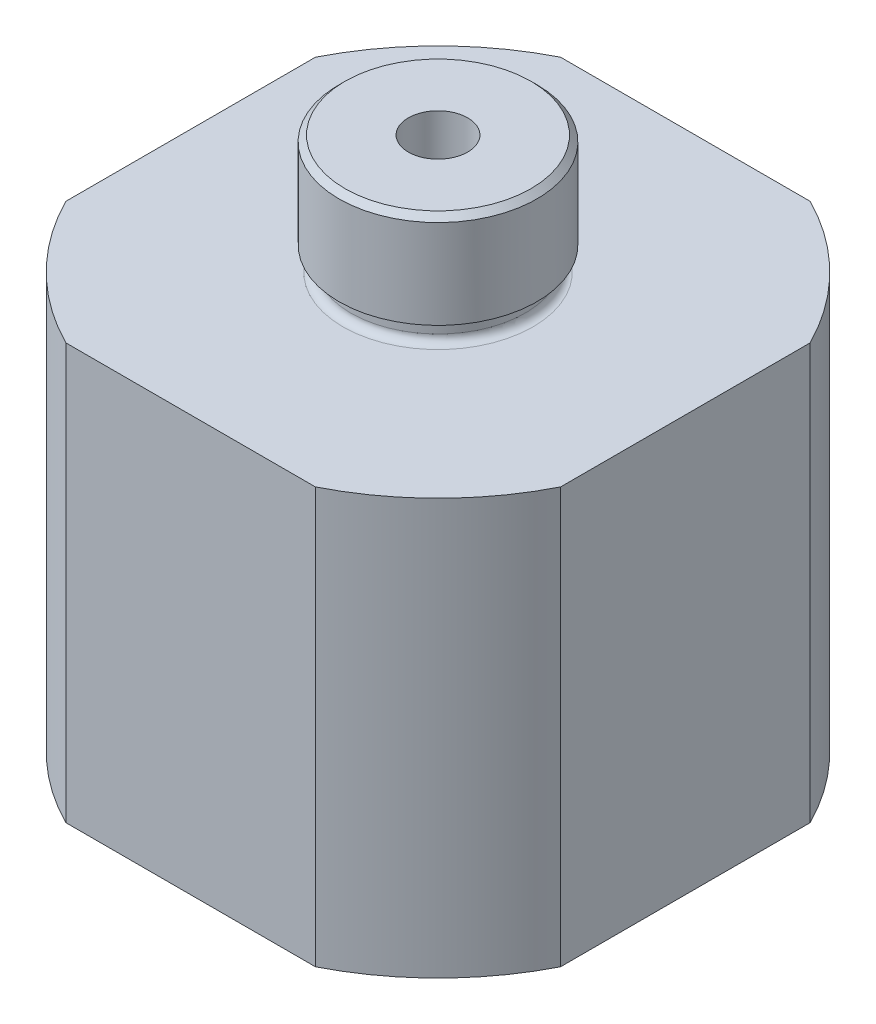
SolidWorks part; units mm, degrees
ref_plane "Front Plane" through (0, 0, 0) normal (0, 0, 1) x (1, 0, 0)
ref_plane "Top Plane" through (0, 0, 0) normal (0, 1, 0) x (1, 0, 0)
ref_plane "Right Plane" through (0, 0, 0) normal (1, 0, 0) x (0, 0, -1)
sketch "Sketch1" plane through (0, 0, 0) normal (0, 0, 1) x (1, 0, 0)
  line L0 (0, 0) -> (-14, 0)
  line L1 (-14, 0) -> (-14, 21)
  line L2 (-14, 21) -> (-4.4, 21)
  line L3 (-4.4, 21) -> (-4.4, 22.2)
  line L4 (-4.4, 22.2) -> (-5, 22.2)
  line L5 (-5, 22.2) -> (-5, 27)
  line L6 (-5, 27) -> (0, 27)
  line L7 (0, 27) -> (0, 0)
  dimension "D1" = 27
  dimension "D2" = 6
  dimension "D3" = 1.2
  dimension "D4" = 5
  dimension "D5" = 14
  dimension "D6" = 4.4
revolve "Revolve1" add sketch "Sketch1" angle 360 about L7
fillet "Fillet1" radius 0.4 2 edges at (0, 22.2, 4.4) (0, 21, 4.4)
sketch "Sketch2" plane through (0, 0, 0) normal (0, -1, 0) x (1, 0, 0)
  circle A0 centre (0, 0) radius 10
  dimension "D1" = 20
extrude "Cut-Extrude1" cut sketch "Sketch2" against normal blind 14
sketch "Sketch3" plane through (0, 14, 0) normal (0, -1, 0) x (1, 0, 0)
  circle A0 centre (0, 0) radius 10.25
  dimension "D1" = 20.5
extrude "Cut-Extrude2" cut sketch "Sketch3" against normal blind 4
sketch "Sketch4" plane through (0, 18, 0) normal (0, -1, 0) x (1, 0, 0)
  circle A0 centre (0, 0) radius 1.5
  dimension "D1" = 3
extrude "Cut-Extrude3" cut sketch "Sketch4" against normal blind 90
chamfer "Chamfer1" distance 0.3 angle 45 1 edges at (0, 27, 5)
chamfer "Chamfer2" distance 1 angle 45 1 edges at (0, 0, -10)
sketch "Sketch5" plane through (0, 21, 0) normal (0, 1, 0) x (1, 0, 0)
  line L1 (12.5, -12.5) -> (-12.5, -12.5)
  line L2 (12.5, -12.5) -> (12.5, 12.5)
  line L3 (12.5, 12.5) -> (-12.5, 12.5)
  line L4 (-12.5, -12.5) -> (-12.5, 12.5)
  line L5 (12.5, -12.5) -> (-12.5, 12.5) construction
  line L6 (12.5, 12.5) -> (-12.5, -12.5) construction
  point P0 (0, 0)
  dimension "D1" = 25
  dimension "D2" = 25
extrude "Cut-Extrude4" cut sketch "Sketch5" against normal blind 90 flip side to cut
